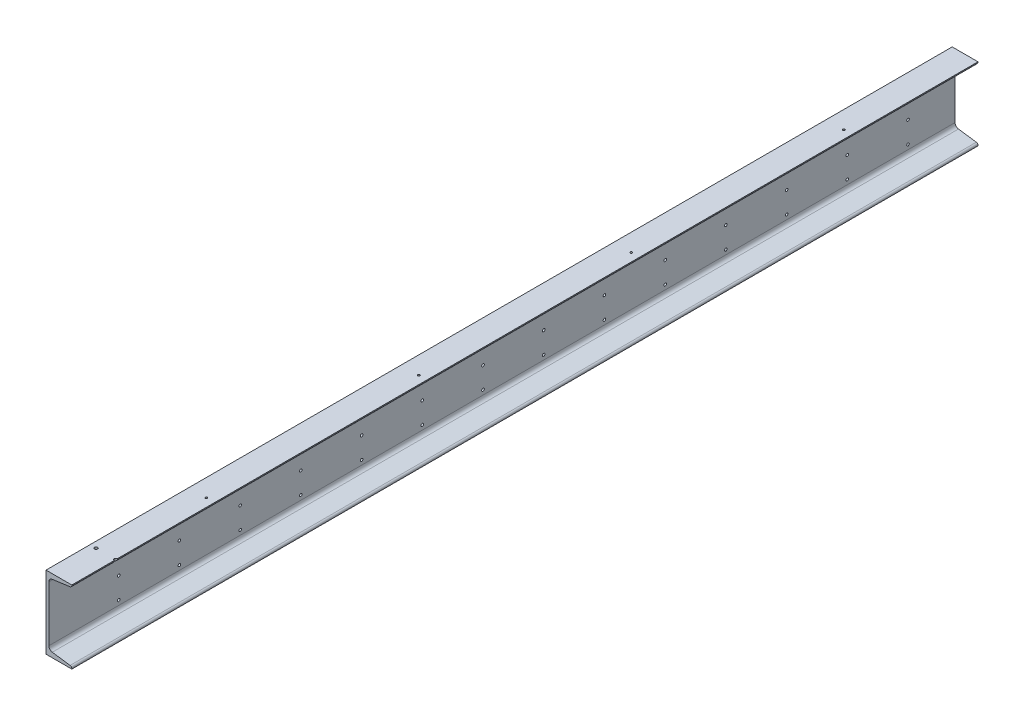
from build123d import *

# Parameters (mm, degrees)
EXTRUDE_1_DEPTH         = 2985
HOLE_WIZARD_M10_2_D     = 8.5
HOLE_WIZARD_M10_2_DEPTH = 24.5
HOLE_WIZARD_M10_2_TIP   = 2.553657631
HOLE_WIZARD_M8_1_D      = 6.8
HOLE_WIZARD_M8_1_DEPTH  = 19.75
HOLE_WIZARD_M8_1_TIP    = 2.042926105
HOLE_WIZARD_M12_1_D     = 10.2
HOLE_WIZARD_M12_1_DEPTH = 29.25
HOLE_WIZARD_M12_1_TIP   = 3.064389157
SKETCH_14_R             = 22.5
CUT_EXTRUDE_1_DEPTH     = 10


with BuildPart() as part:
    # 草图1 → 凸台-拉伸1 (new body)
    with BuildSketch(Plane.XY):
        with BuildLine():
            Line((0, 0), (-85, 0))
            Line((-85, 0), (-85, -240))
            Line((-85, -240), (0, -240))
            Line((0, -240), (0, -238.623349271))
            ThreePointArc((0, -238.623349271), (-1.594387729, -234.358965582), (-5.595374844, -232.186606824))
            Line((-5.595374844, -232.186606824), (-64.309250312, -223.934909757))
            ThreePointArc((-64.309250312, -223.934909757), (-72.311224543, -219.59019224), (-75.5, -211.061424863))
            Line((-75.5, -211.061424863), (-75.5, -28.938575137))
            ThreePointArc((-75.5, -28.938575137), (-72.311224543, -20.40980776), (-64.309250312, -16.065090243))
            Line((-64.309250312, -16.065090243), (-5.595374844, -7.813393176))
            ThreePointArc((-5.595374844, -7.813393176), (-1.594387729, -5.641034418), (0, -1.376650729))
            Line((0, -1.376650729), (0, 0))
        make_face()
    extrude(amount=EXTRUDE_1_DEPTH)

    # M10 螺纹孔2
    with Locations(Plane.ZY.offset(85)):
        with Locations((155, -126), (155, -196), (355, -126), (355, -196), (555, -126), (555, -196), (755, -126), (755, -196), (955, -126), (955, -196), (1155, -126), (1155, -196), (1355, -126), (1355, -196), (1555, -196), (1555, -126), (1755, -196), (1755, -126), (1955, -126), (1955, -196), (2155, -196), (2155, -126), (2355, -126), (2355, -196), (2555, -196), (2555, -126), (2755, -126), (2755, -196)):
            Hole(HOLE_WIZARD_M10_2_D / 2, depth=HOLE_WIZARD_M10_2_DEPTH)
            with Locations((0, 0, -(HOLE_WIZARD_M10_2_DEPTH + HOLE_WIZARD_M10_2_TIP / 2))):  # 118° drill point
                Cone(0, HOLE_WIZARD_M10_2_D / 2, HOLE_WIZARD_M10_2_TIP, mode=Mode.SUBTRACT)

    # M8 螺纹孔1
    with Locations(Plane(origin=(0, 0, 0), x_dir=(1, 0, 0), z_dir=(0, 1, 0))):
        with Locations((-27, -415), (-27, -1115), (-27, -1815), (-27, -2515)):
            Hole(HOLE_WIZARD_M8_1_D / 2, depth=HOLE_WIZARD_M8_1_DEPTH)
            with Locations((0, 0, -(HOLE_WIZARD_M8_1_DEPTH + HOLE_WIZARD_M8_1_TIP / 2))):  # 118° drill point
                Cone(0, HOLE_WIZARD_M8_1_D / 2, HOLE_WIZARD_M8_1_TIP, mode=Mode.SUBTRACT)

    # M12 螺纹孔1
    with Locations(Plane(origin=(0, 0, 0), x_dir=(1, 0, 0), z_dir=(0, 1, 0))):
        with Locations((-65, -2840), (0, -2840)):
            Hole(HOLE_WIZARD_M12_1_D / 2, depth=HOLE_WIZARD_M12_1_DEPTH)
            with Locations((0, 0, -(HOLE_WIZARD_M12_1_DEPTH + HOLE_WIZARD_M12_1_TIP / 2))):  # 118° drill point
                Cone(0, HOLE_WIZARD_M12_1_D / 2, HOLE_WIZARD_M12_1_TIP, mode=Mode.SUBTRACT)

    # 草图14 → 切除-拉伸1 (cut)
    with BuildSketch(Plane.ZY.offset(85)):
        with Locations(Location((1600, -50, 0), (0, 0, 270))):
            Circle(SKETCH_14_R)
    extrude(amount=-CUT_EXTRUDE_1_DEPTH, mode=Mode.SUBTRACT)


solid = part.part
